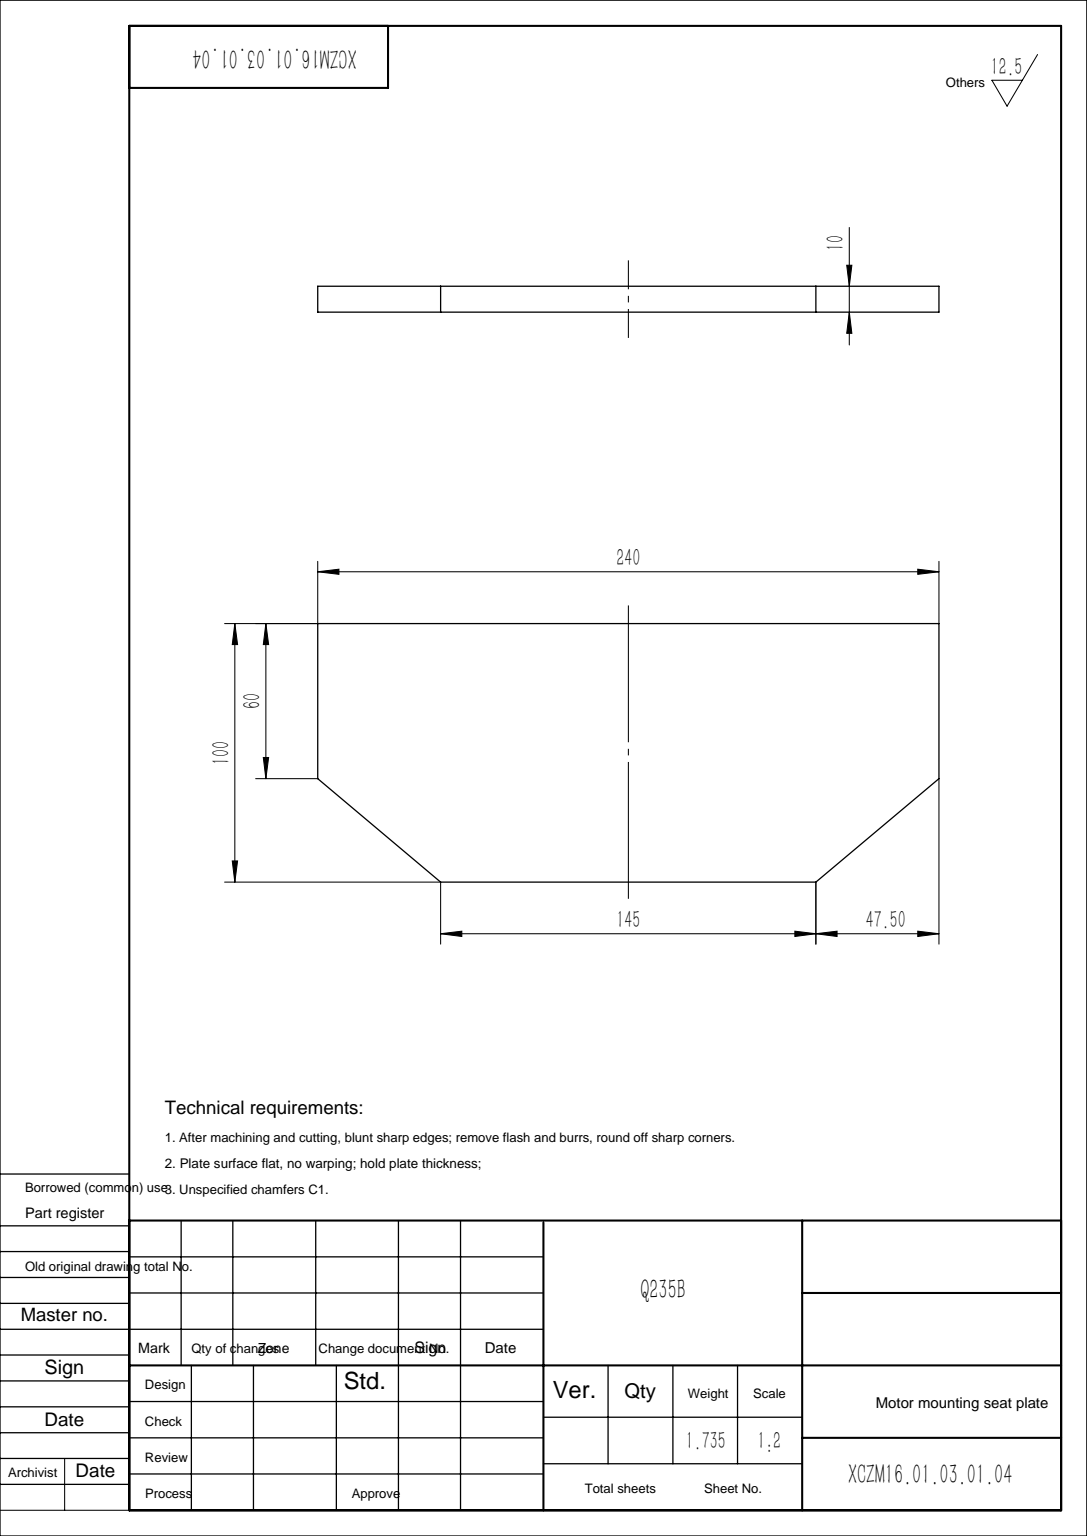
from build123d import *

# Parameters (mm, degrees)
EXTRUDE_1_DEPTH = 10


with BuildPart() as part:
    # 草图1 → 凸台-拉伸1 (new body)
    with BuildSketch(Plane.XY):
        Polygon((120, 0), (-120, 0), (-120, -60), (-72.5, -100), (72.5, -100), (120, -60), align=None)
    extrude(amount=EXTRUDE_1_DEPTH)


solid = part.part
